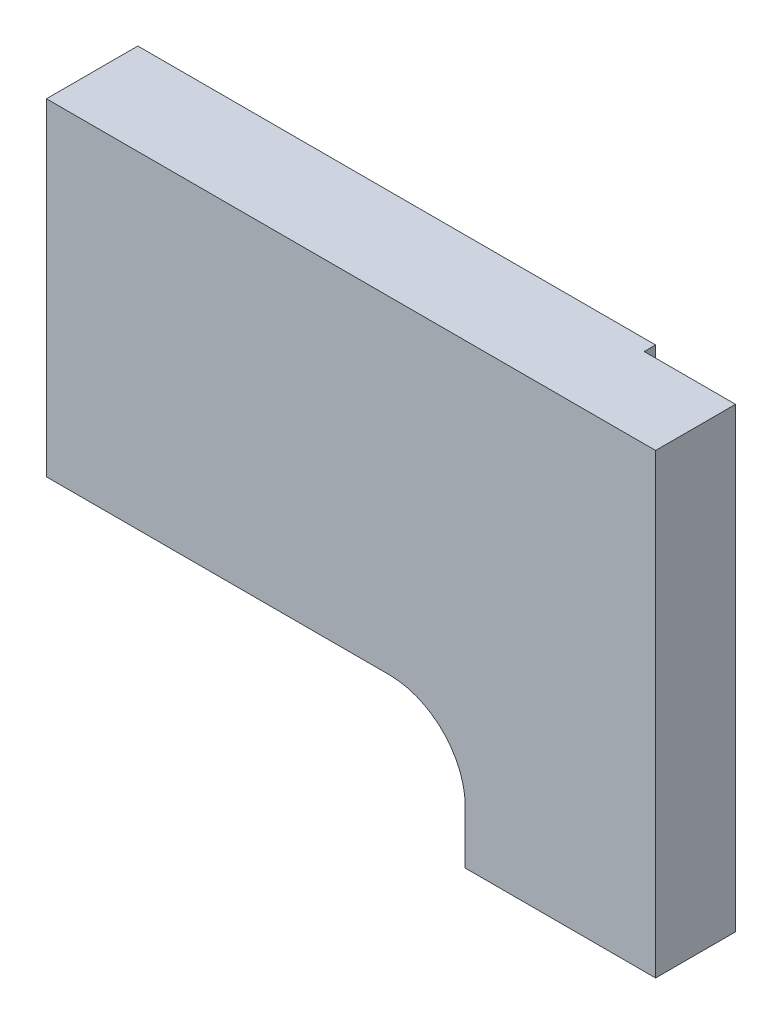
SolidWorks part; units mm, degrees
ref_plane "前视基准面" through (0, 0, 0) normal (0, 0, 1) x (1, 0, 0)
ref_plane "上视基准面" through (0, 0, 0) normal (0, 1, 0) x (1, 0, 0)
ref_plane "右视基准面" through (0, 0, 0) normal (1, 0, 0) x (0, 0, -1)
sketch "草图1" plane through (0, 0, 0) normal (0, 0, 1) x (1, 0, 0)
  line L1 (-40, -30) -> (40, -30)
  line L2 (-40, -30) -> (-40, 30)
  line L3 (-40, 30) -> (40, 30)
  line L4 (40, -30) -> (40, 30)
  line L5 (-40, -30) -> (40, 30) construction
  line L6 (-40, 30) -> (40, -30) construction
  point P0 (0, 0)
  dimension "D1" = 60
  dimension "D2" = 80
extrude "凸台-拉伸1" add sketch "草图1" along normal mid plane 12
sketch "草图2" plane through (0, 0, -6) normal (0, 0, 1) x (1, 0, 0)
  line L0 (-40, -30) -> (40, -30) construction
  line L1 (40, 30) -> (28, 30)
  line L2 (40, 30) -> (40, -30)
  line L3 (40, -30) -> (28, -30)
  line L4 (28, 30) -> (28, -30)
  dimension "D1" = 12
extrude "切除-拉伸1" cut sketch "草图2" along normal blind 1.5
sketch "草图3" plane through (0, 0, -6) normal (0, 0, -1) x (-1, 0, 0)
  line L0 (-28, 30) -> (40, 30) construction
  line L1 (40, -30) -> (-15, -30)
  line L2 (40, -30) -> (40, -13)
  line L3 (40, -13) -> (-15, -13)
  line L4 (-15, -30) -> (-15, -13)
  dimension "D1" = 43
  dimension "D2" = 55
extrude "切除-拉伸2" cut sketch "草图3" against normal up to next
fillet "圆角1" radius 10 1 edges at (15, -13, 0)
